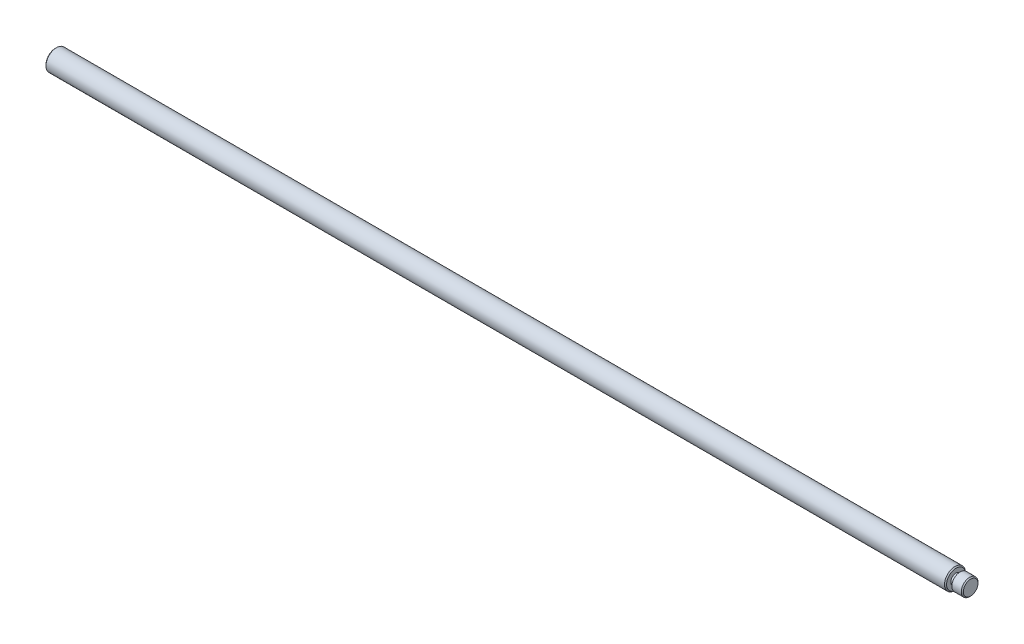
from build123d import *

# Parameters (mm, degrees)
SKETCH1_R           = 5
BOSS_EXTRUDE1_DEPTH = 215
SKETCH2_R           = 2.5
BOSS_EXTRUDE2_DEPTH = 2
SKETCH3_R           = 4
BOSS_EXTRUDE3_DEPTH = 5
CHAMFER1_SIZE       = 0.5


with BuildPart() as part:
    # Sketch1 → Boss-Extrude1 (new, symmetric)
    with BuildSketch(Plane(origin=(0, 0, 0), x_dir=(0, 0, -1), z_dir=(1, 0, 0))):
        Circle(SKETCH1_R)
    extrude(amount=BOSS_EXTRUDE1_DEPTH, both=True)

    # Sketch2 → Boss-Extrude2 (add)
    with BuildSketch(Plane(origin=(215, 0, 0), x_dir=(0, 0, -1), z_dir=(1, 0, 0))):
        Circle(SKETCH2_R)
    extrude(amount=BOSS_EXTRUDE2_DEPTH)

    # Sketch3 → Boss-Extrude3 (add)
    with BuildSketch(Plane(origin=(217, 0, 0), x_dir=(0, 0, -1), z_dir=(1, 0, 0))):
        Circle(SKETCH3_R)
    extrude(amount=BOSS_EXTRUDE3_DEPTH)

    # Chamfer1
    chamfer1_edges = [part.edges().sort_by_distance(p)[0] for p in [
        (-215, 0, 5),
        (215, 0, 5),
        (222, 0, 4),
    ]]
    chamfer(chamfer1_edges, length=CHAMFER1_SIZE)


solid = part.part
